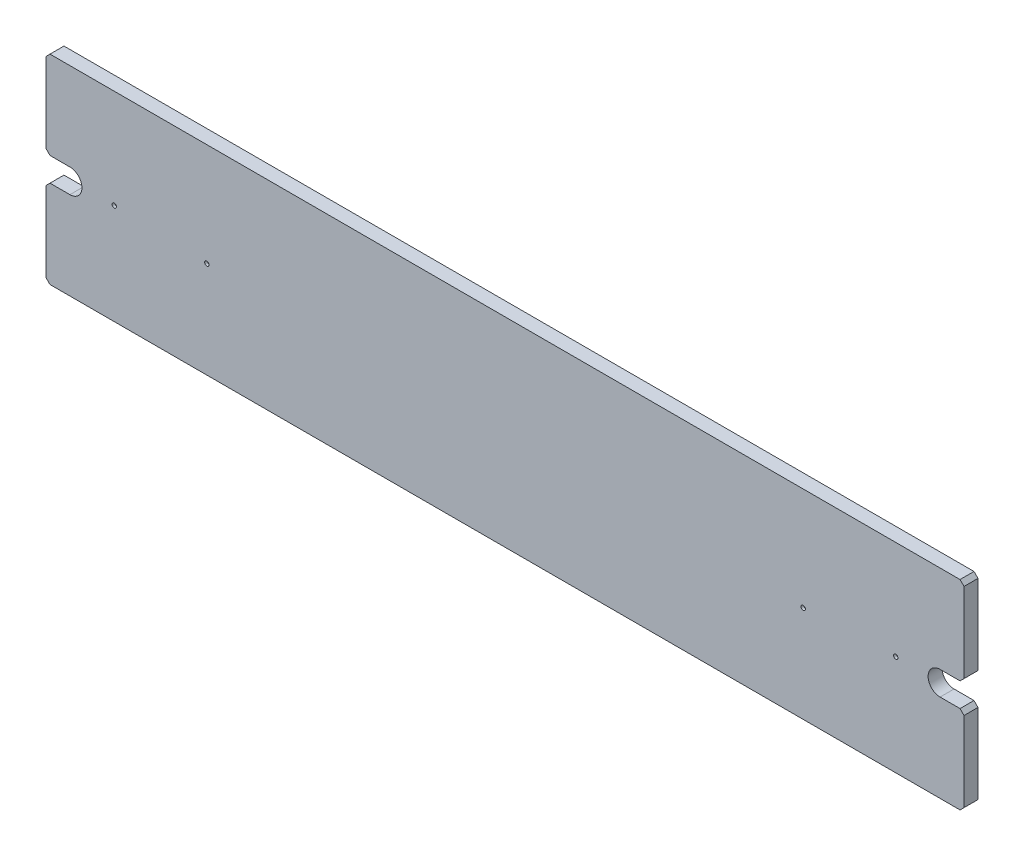
from build123d import *

# Parameters (mm, degrees)
SKETCH1_W                                            = 2300
SKETCH1_H                                            = 500
BOSS_EXTRUDE1_DEPTH                                  = 35
SKETCH2_R                                            = 40
CUT_EXTRUDE1_DEPTH                                   = 5
BOSS_EXTRUDE2_DEPTH                                  = 5
SKETCH4_R                                            = 2.5
CUT_EXTRUDE2_DEPTH                                   = 5
CUT_EXTRUDE3_DEPTH                                   = 1178.380567191
CHAMFER1_SIZE                                        = 10
SKETCH7_R                                            = 40
CUT_EXTRUDE4_DEPTH                                   = 5
CBORE_FOR_M6_HEXAGON_SOCKET_HEAD_CAP_SCR_D           = 6.6
CBORE_FOR_M6_HEXAGON_SOCKET_HEAD_CAP_SCR_CBORE_D     = 11
CBORE_FOR_M6_HEXAGON_SOCKET_HEAD_CAP_SCR_CBORE_DEPTH = 6.8
M8_TAPPED_HOLE1_D                                    = 6.8
M8_TAPPED_HOLE1_DEPTH                                = 19
M8_TAPPED_HOLE1_TIP                                  = 2.042926105


with BuildPart() as part:
    # Sketch1 → Boss-Extrude1 (new body)
    with BuildSketch(Plane.XY):
        Rectangle(SKETCH1_W, SKETCH1_H)
    extrude(amount=BOSS_EXTRUDE1_DEPTH)

    # Sketch2 → Cut-Extrude1 (cut)
    with BuildSketch(Plane(origin=(0, 0, 0), x_dir=(-1, 0, 0), z_dir=(0, 0, -1))):
        with Locations((-979, 2)):
            Circle(SKETCH2_R)
        with Locations((979, 2)):
            Circle(SKETCH2_R)
    extrude(amount=-CUT_EXTRUDE1_DEPTH, mode=Mode.SUBTRACT)

    # Sketch3 → Boss-Extrude2 (add)
    with BuildSketch(Plane(origin=(0, 0, 0), x_dir=(-1, 0, 0), z_dir=(0, 0, -1))):
        with BuildLine():
            Line((-947, -22), (-947, 26))
            ThreePointArc((-947, 26), (-939, 2), (-947, -22))
        make_face()
        with BuildLine():
            Line((947, -22), (947, 26))
            ThreePointArc((947, 26), (939, 2), (947, -22))
        make_face()
    extrude(amount=-BOSS_EXTRUDE2_DEPTH)

    # Sketch4 → Cut-Extrude2 (cut)
    with BuildSketch(Plane(origin=(0, 0, 5), x_dir=(-1, 0, 0), z_dir=(0, 0, -1))):
        with Locations((-947, -22)):
            Circle(SKETCH4_R)
        with Locations((-947, 26)):
            Circle(SKETCH4_R)
        with Locations((947, -22)):
            Circle(SKETCH4_R)
        with Locations((947, 26)):
            Circle(SKETCH4_R)
    extrude(amount=CUT_EXTRUDE2_DEPTH, mode=Mode.SUBTRACT)

    # Sketch6 → Cut-Extrude3 (cut, through all)
    with BuildSketch(Plane(origin=(0, 0, 0), x_dir=(-1, 0, 0), z_dir=(0, 0, -1))):
        with BuildLine():
            Line((1090, 30), (1190, 30))
            ThreePointArc((1190, 30), (1220, 0), (1190, -30))
            Line((1190, -30), (1090, -30))
            ThreePointArc((1090, -30), (1060, 0), (1090, 30))
        make_face()
        with BuildLine():
            Line((-1090, 30), (-1190, 30))
            ThreePointArc((-1190, 30), (-1220, 0), (-1190, -30))
            Line((-1190, -30), (-1090, -30))
            ThreePointArc((-1090, -30), (-1060, 0), (-1090, 30))
        make_face()
    extrude(amount=-CUT_EXTRUDE3_DEPTH, mode=Mode.SUBTRACT)

    # Chamfer1
    chamfer1_edges = [part.edges().sort_by_distance(p)[0] for p in [
        (-1150, 30, 17.5),
        (-1150, -30, 17.5),
        (1150, -30, 17.5),
        (1150, 30, 17.5),
        (1150, -250, 17.5),
        (-1150, -250, 17.5),
        (-1150, 250, 17.5),
        (1150, 250, 17.5),
    ]]
    chamfer(chamfer1_edges, length=CHAMFER1_SIZE)

    # Sketch7 → Cut-Extrude4 (cut)
    with BuildSketch(Plane(origin=(0, 0, 0), x_dir=(-1, 0, 0), z_dir=(0, 0, -1))):
        with Locations((340, -76)):
            Circle(SKETCH7_R)
        with Locations((397, 50)):
            Circle(SKETCH7_R)
        with Locations((-2.9799995, 46)):
            Circle(SKETCH7_R)
        with Locations((40, -76)):
            Circle(SKETCH7_R)
        with Locations((-259.958330439, -71)):
            Circle(SKETCH7_R)
        with Locations((-397, 46)):
            Circle(SKETCH7_R)
    extrude(amount=-CUT_EXTRUDE4_DEPTH, mode=Mode.SUBTRACT)

    # CBORE for M6 Hexagon socket head cap screws1 (through all)
    with Locations(Plane.XY.offset(35)):
        with Locations((-747, -8), (747, -8), (-979, 2), (979, 2)):
            CounterBoreHole(CBORE_FOR_M6_HEXAGON_SOCKET_HEAD_CAP_SCR_D / 2, CBORE_FOR_M6_HEXAGON_SOCKET_HEAD_CAP_SCR_CBORE_D / 2, CBORE_FOR_M6_HEXAGON_SOCKET_HEAD_CAP_SCR_CBORE_DEPTH)

    # M8 Tapped Hole1
    with Locations(Plane(origin=(0, 0, 0), x_dir=(-1, 0, 0), z_dir=(0, 0, -1))):
        with Locations((735.5, -125), (595.5, -125), (735.5, 124), (595.5, 124), (-604.5, -125), (-744.5, -125), (-604.5, 124), (-744.5, 124)):
            Hole(M8_TAPPED_HOLE1_D / 2, depth=M8_TAPPED_HOLE1_DEPTH)
            with Locations((0, 0, -(M8_TAPPED_HOLE1_DEPTH + M8_TAPPED_HOLE1_TIP / 2))):  # 118° drill point
                Cone(0, M8_TAPPED_HOLE1_D / 2, M8_TAPPED_HOLE1_TIP, mode=Mode.SUBTRACT)


solid = part.part
